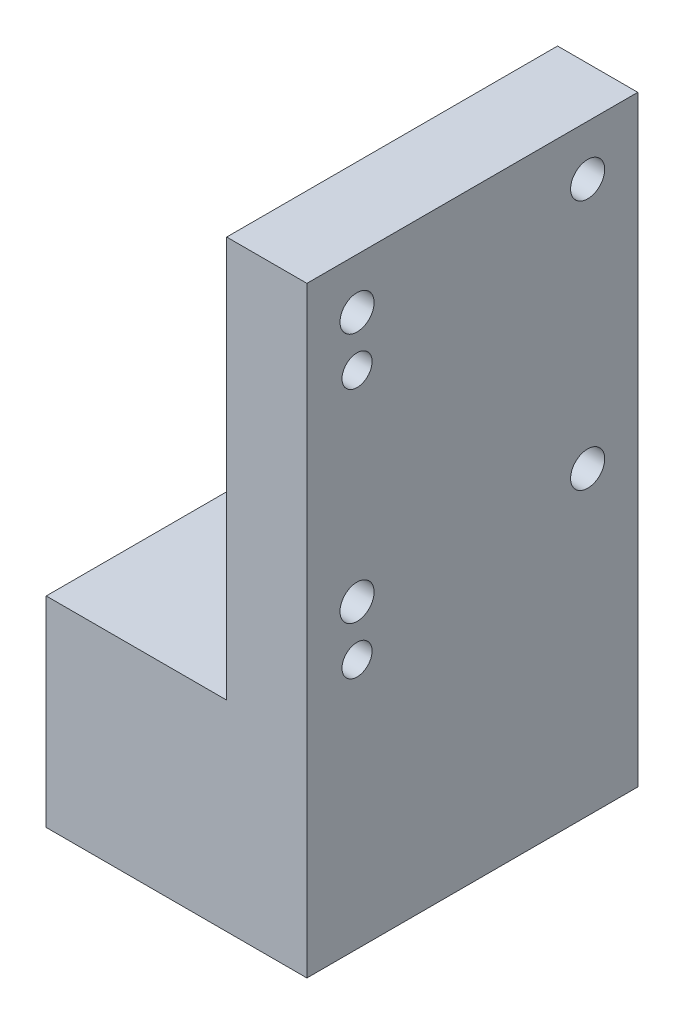
from build123d import *

# Parameters (mm, degrees)
SKETCH_1_W                                        = 33
SKETCH_1_H                                        = 60
BOSS_EXTRUDE_1_DEPTH                              = 8
SKETCH_2_W                                        = 33
SKETCH_2_H                                        = 25
BOSS_EXTRUDE_2_DEPTH                              = 18
M3_HEX_SOCKET_CAP_SCREW_COUNTERBORE_1_D           = 3.4
M3_HEX_SOCKET_CAP_SCREW_COUNTERBORE_1_CBORE_D     = 6.5
M3_HEX_SOCKET_CAP_SCREW_COUNTERBORE_1_CBORE_DEPTH = 3
LINEAR_PATTERN_1_COUNT                            = 2
LINEAR_PATTERN_1_PITCH                            = 23
LINEAR_PATTERN_1_COUNT_DIR2                       = 2
LINEAR_PATTERN_1_PITCH_DIR2                       = 25
LINEAR_PATTERN_2_COUNT                            = 2
LINEAR_PATTERN_2_PITCH                            = 10
SKETCH_9_W                                        = 33
SKETCH_9_H                                        = 5
CUT_EXTRUDE_1_DEPTH                               = 18
F_3_0_3_HOLE_1_D                                  = 3
LINEAR_PATTERN_3_COUNT                            = 2
LINEAR_PATTERN_3_PITCH                            = 25
LINEAR_PATTERN_4_COUNT                            = 2
LINEAR_PATTERN_4_PITCH                            = 16


with BuildPart() as part:
    # Sketch 1 → Boss-Extrude 1 (new body)
    with BuildSketch(Plane(origin=(0, 0, 0), x_dir=(0, 0, -1), z_dir=(1, 0, 0))):
        Rectangle(SKETCH_1_W, SKETCH_1_H)
    extrude(amount=BOSS_EXTRUDE_1_DEPTH)

    # Sketch 2 → Boss-Extrude 2 (add)
    with BuildSketch(Plane.ZY):
        with Locations((0, -17.5)):
            Rectangle(SKETCH_2_W, SKETCH_2_H)
    extrude(amount=BOSS_EXTRUDE_2_DEPTH)

    # M3 Hex Socket Cap Screw Counterbore 1 (through all)
    with Locations(Plane.ZY):
        with Locations((-11.5, 25)):
            m3_hex_socket_cap_screw_counterbore_1 = CounterBoreHole(M3_HEX_SOCKET_CAP_SCREW_COUNTERBORE_1_D / 2, M3_HEX_SOCKET_CAP_SCREW_COUNTERBORE_1_CBORE_D / 2, M3_HEX_SOCKET_CAP_SCREW_COUNTERBORE_1_CBORE_DEPTH)

    # Linear Pattern 1: M3 Hex Socket Cap Screw Counterbore 1 2 × 2
    with Locations(*[(0, -j * LINEAR_PATTERN_1_PITCH_DIR2, i * LINEAR_PATTERN_1_PITCH) for i in range(LINEAR_PATTERN_1_COUNT) for j in range(LINEAR_PATTERN_1_COUNT_DIR2) if (i, j) != (0, 0)]):
        add(m3_hex_socket_cap_screw_counterbore_1, mode=Mode.SUBTRACT)

    # Sketch 7 → M4 Tapped Hole 2 (revolve, cut)
    with BuildSketch(Plane(origin=(-18, -25, 0), x_dir=(0, 0, 1), z_dir=(0, 1, 0))):
        Polygon((0, 0), (0, 11.091420021), (1.65, 10.1), (1.65, 0), align=None)
    m4_tapped_hole_2 = revolve(axis=Axis((-24.35, -25, 0), (1, 0, 0)), mode=Mode.SUBTRACT)

    # Linear Pattern 2: M4 Tapped Hole 2 ×2
    with Locations(*[(0, i * LINEAR_PATTERN_2_PITCH, 0) for i in range(1, LINEAR_PATTERN_2_COUNT)]):
        add(m4_tapped_hole_2, mode=Mode.SUBTRACT)

    # Sketch 9 → Cut-Extrude 1 (cut)
    with BuildSketch(Plane.ZY.offset(18)):
        with Locations((0, -7.5)):
            Rectangle(SKETCH_9_W, SKETCH_9_H)
    extrude(amount=-CUT_EXTRUDE_1_DEPTH, mode=Mode.SUBTRACT)

    # Ø3.0 (3) Hole 1 (through all)
    with Locations(Plane.ZY):
        with Locations((11.5, 20)):
            f_3_0_3_hole_1 = Hole(F_3_0_3_HOLE_1_D / 2)

    # Linear Pattern 3: Ø3.0 (3) Hole 1 ×2
    with Locations(*[(0, -i * LINEAR_PATTERN_3_PITCH, 0) for i in range(1, LINEAR_PATTERN_3_COUNT)]):
        add(f_3_0_3_hole_1, mode=Mode.SUBTRACT)

    # Sketch 12 → Ø4.0 (4) Hole 1 (revolve, cut)
    with BuildSketch(Plane(origin=(-18, -20, -8), x_dir=(0, 0, 1), z_dir=(0, 1, 0))):
        Polygon((0, 0), (0, 11.201721238), (2, 10), (2, 0), align=None)
    f_4_0_4_hole_1 = revolve(axis=Axis((-24.35, -20, -8), (1, 0, 0)), mode=Mode.SUBTRACT)

    # Linear Pattern 4: Ø4.0 (4) Hole 1 ×2
    with Locations(*[(0, 0, i * LINEAR_PATTERN_4_PITCH) for i in range(1, LINEAR_PATTERN_4_COUNT)]):
        add(f_4_0_4_hole_1, mode=Mode.SUBTRACT)


solid = part.part
